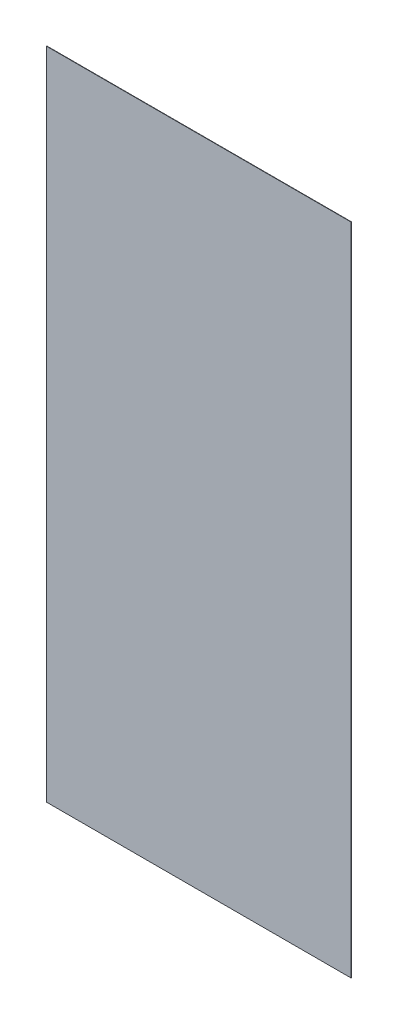
SolidWorks part; units mm, degrees
material "Q235B"
ref_plane "Front Plane" through (0, 0, 0) normal (0, 0, 1) x (1, 0, 0)
ref_plane "Top Plane" through (0, 0, 0) normal (0, 1, 0) x (1, 0, 0)
ref_plane "Right Plane" through (0, 0, 0) normal (1, 0, 0) x (0, 0, -1)
sketch "Sketch1" plane through (0, 0, 0) normal (0, 0, 1) x (1, 0, 0)
  line L1 (400, -860) -> (-400, -860)
  line L2 (400, -860) -> (400, 860)
  line L3 (400, 860) -> (-400, 860)
  line L4 (-400, -860) -> (-400, 860)
  line L5 (400, -860) -> (-400, 860) construction
  line L6 (400, 860) -> (-400, -860) construction
  point P0 (0, 0)
  dimension "D1" = 1720
  dimension "D2" = 800
extrude "Boss-Extrude1" add sketch "Sketch1" along normal blind 1
